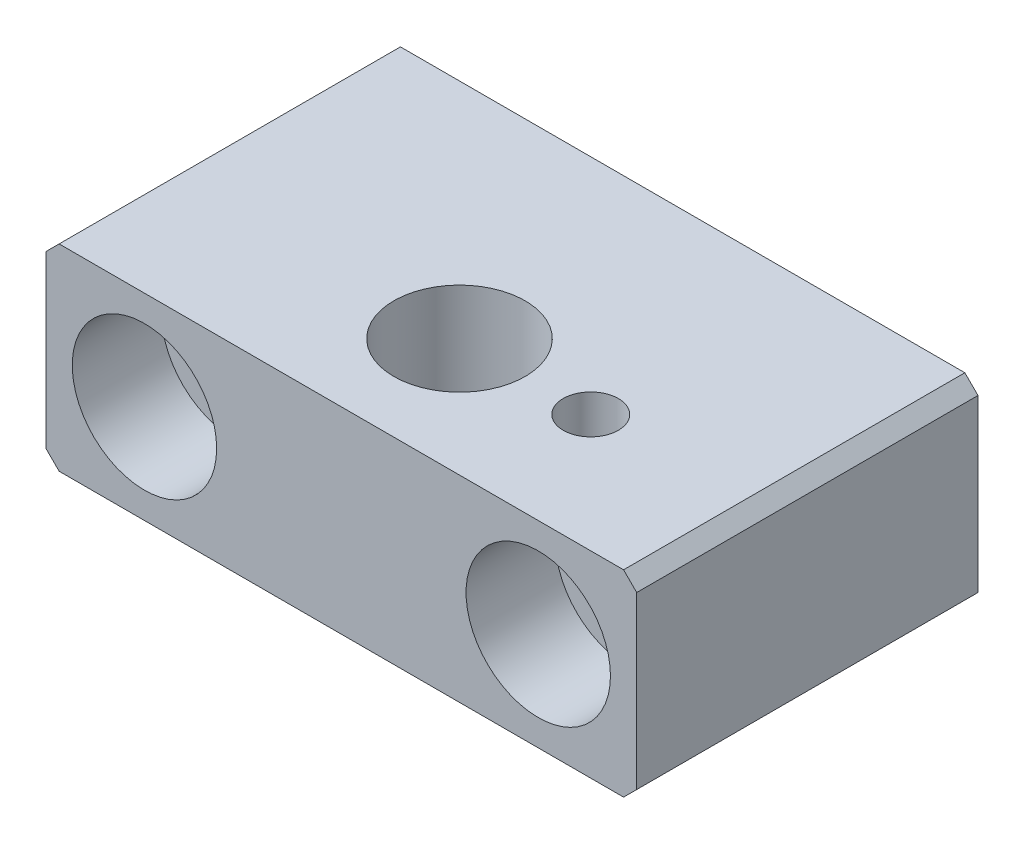
SolidWorks part; units mm, degrees
material "S45C"
ref_plane "Front" through (0, 0, 0) normal (0, 0, 1) x (1, 0, 0)
ref_plane "Top" through (0, 0, 0) normal (0, 1, 0) x (1, 0, 0)
ref_plane "Right" through (0, 0, 0) normal (1, 0, 0) x (0, 0, -1)
sketch "Sketch1" plane through (0, 0, 0) normal (0, 1, 0) x (1, 0, 0)
  line L1 (-22.5, 13) -> (22.5, 13)
  line L2 (-22.5, 13) -> (-22.5, -13)
  line L3 (-22.5, -13) -> (22.5, -13)
  line L4 (22.5, 13) -> (22.5, -13)
  line L5 (-22.5, 13) -> (22.5, -13) construction
  line L6 (-22.5, -13) -> (22.5, 13) construction
  point P0 (0, 0)
  dimension "D1" = 26
  dimension "D2" = 45
extrude "Boss-Extrude1" add sketch "Sketch1" along normal blind 15
sketch "Sketch2" plane through (0, 15, 0) normal (0, 1, 0) x (1, 0, 0)
  circle A0 centre (0, -4) radius 5
  dimension "D1" = 10
extrude "Cut-Extrude1" cut sketch "Sketch2" against normal through all
hole_wizard "Ø6.0mm Dowel Hole 1" positions "Sketch5" profile "Sketch4" hole size "Ø6.0" standard "GB"
sketch "Sketch5" plane through (0, 0, -13) normal (0, 0, -1) x (-1, 0, 0)
  line L0 (-22.5, 7.5) -> (22.5, 7.5) construction
  line L1 (-22.5, 15) -> (-22.5, 0) construction
  line L2 (22.5, 15) -> (22.5, 0) construction
  line L4 (0, 0) -> (0, 15) construction
  line L5 (-22.5, 15) -> (22.5, 15) construction
  point P15 (5, 7.5)
  point P17 (-5, 7.5)
  dimension "D1" = 10
sketch "Sketch4" plane through (5, 7.5, -13) normal (1, 0, 0) x (0, 1, 0)
  line L0 (0, 0) -> (0, 11.8026)
  line L1 (0, 11.8026) -> (3, 10)
  line L2 (3, 10) -> (3, 0)
  line L5 (3, 0) -> (0, 0)
  line L10 (0, 11.8026) -> (-3, 10) construction
  line L11 (0, -6.35) -> (0, 107.95) construction
  dimension "孔直径" = 6
  dimension "孔深度" = 10
  dimension "导头角度" = 118
chamfer "Chamfer1" distance 1 angle 45 4 edges at (22.5, 0, 0) (22.5, 15, 0) (-22.5, 0, 0) (-22.5, 15, 0)
hole_wizard "CBORE for M6 Hexagon socket head cap screws1" positions "Sketch8" profile "Sketch7" counterbore size "M6" standard "GB" end condition through all
sketch "Sketch8" plane through (0, 0, 13) normal (0, 0, 1) x (1, 0, 0)
  line L0 (0, 0) -> (0, 15) construction
  line L1 (-21.5, 15) -> (21.5, 15) construction
  line L3 (-22.5, 7.5) -> (22.5, 7.5) construction
  line L4 (-22.5, 14) -> (-22.5, 1) construction
  line L5 (22.5, 14) -> (22.5, 1) construction
  point P15 (15, 7.5)
  point P17 (-15, 7.5)
  dimension "D1" = 30
sketch "Sketch7" plane through (-15, 7.5, 13) normal (1, 0, 0) x (0, -1, 0)
  line L0 (0, 0) -> (0, 26)
  line L1 (0, 26) -> (3.3, 26)
  line L3 (3.3, 26) -> (3.3, 6.8)
  line L4 (3.3, 6.8) -> (5.5, 6.8)
  line L5 (5.5, 6.8) -> (5.5, 0)
  line L7 (5.5, 0) -> (0, 0)
  line L11 (0, -6.35) -> (0, 107.95) construction
  dimension "通孔孔直径" = 6.6
  dimension "通孔孔深度" = 26
  dimension "柱形沉头孔直径" = 11
  dimension "柱形沉头孔深度" = 6.8
hole_wizard "M5 Tapped Hole1" positions "Sketch11" profile "Sketch10" tap size "M5" standard "GB"
sketch "Sketch11" plane through (0, 15, 0) normal (0, 1, 0) x (1, 0, 0)
  line L0 (0, -4) -> (22.5, -4) construction
  line L1 (22.5, 13) -> (22.5, -13) construction
  point P10 (10, -4)
  dimension "D1" = 10
sketch "Sketch10" plane through (10, 15, 4) normal (1, 0, 0) x (0, 0, 1)
  line L0 (0, 0) -> (0, 15.2618)
  line L1 (0, 15.2618) -> (2.1, 14)
  line L2 (2.1, 14) -> (2.1, 0)
  line L5 (2.1, 0) -> (0, 0)
  line L10 (0, 15.2618) -> (-2.1, 14) construction
  line L11 (0, -6.35) -> (0, 107.95) construction
  dimension "螺纹孔钻头直径" = 4.2
  dimension "螺纹孔钻头深度" = 14
  dimension "导头角度" = 118
cosmetic thread "Tapped Hole 1" parameters "D1"=10, "D2"=5
